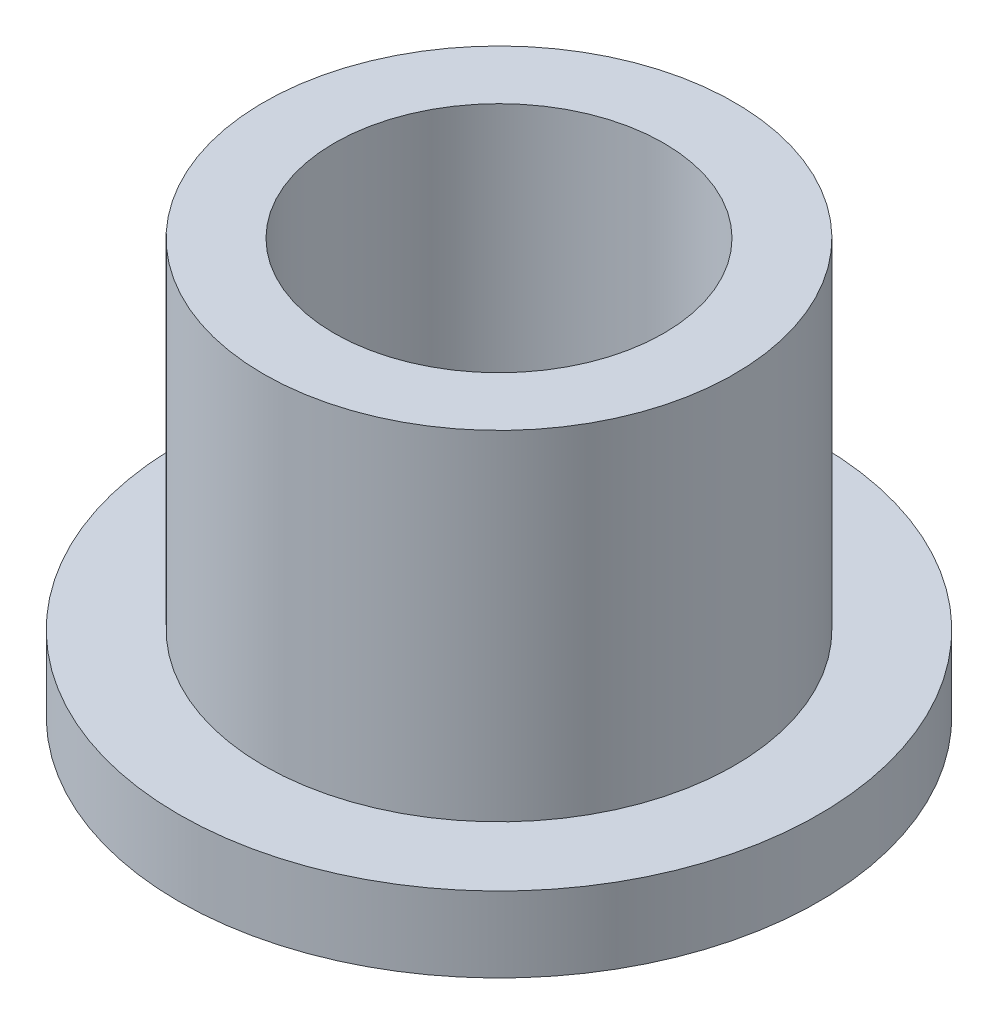
from build123d import *

# Parameters (mm, degrees)
SKETCH1_R           = 34
BOSS_EXTRUDE1_DEPTH = 8
SKETCH2_R           = 25
BOSS_EXTRUDE2_DEPTH = 36
SKETCH3_R           = 17.5
CUT_EXTRUDE1_DEPTH  = 66.176682947


with BuildPart() as part:
    # Sketch1 → Boss-Extrude1 (new body)
    with BuildSketch(Plane(origin=(0, 0, 0), x_dir=(1, 0, 0), z_dir=(0, 1, 0))):
        with Locations(Location((0, 0, 0), (0, 0, 270))):
            Circle(SKETCH1_R)
    extrude(amount=BOSS_EXTRUDE1_DEPTH)

    # Sketch2 → Boss-Extrude2 (add)
    with BuildSketch(Plane(origin=(0, 8, 0), x_dir=(1, 0, 0), z_dir=(0, 1, 0))):
        with Locations(Location((0, 0, 0), (0, 0, 270))):
            Circle(SKETCH2_R)
    extrude(amount=BOSS_EXTRUDE2_DEPTH)

    # Sketch3 → Cut-Extrude1 (cut, through all)
    with BuildSketch(Plane(origin=(0, 44, 0), x_dir=(1, 0, 0), z_dir=(0, 1, 0))):
        with Locations(Location((0, 0, 0), (0, 0, 270))):
            Circle(SKETCH3_R)
    extrude(amount=-CUT_EXTRUDE1_DEPTH, mode=Mode.SUBTRACT)


solid = part.part
